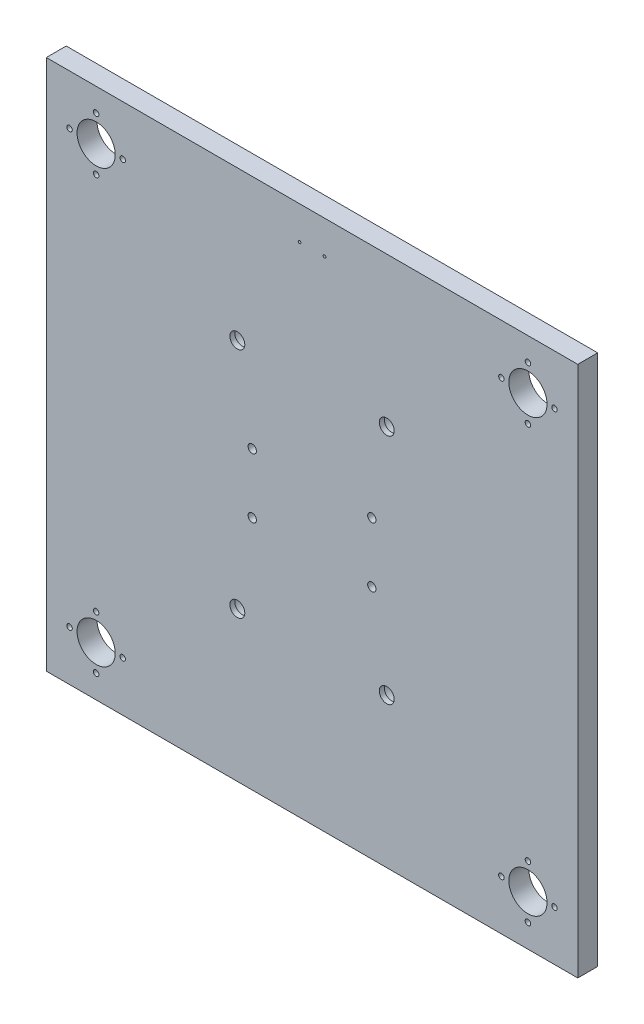
SolidWorks part; units mm, degrees
material "6061 合金"
ref_plane "前视基准面" through (0, 0, 0) normal (0, 0, 1) x (1, 0, 0)
ref_plane "上视基准面" through (0, 0, 0) normal (0, 1, 0) x (1, 0, 0)
ref_plane "右视基准面" through (0, 0, 0) normal (1, 0, 0) x (0, 0, -1)
sketch "草图1" plane through (0, 0, 0) normal (0, 0, 1) x (1, 0, 0)
  line L1 (-160, 160) -> (160, 160)
  line L2 (-160, 160) -> (-160, -160)
  line L3 (-160, -160) -> (160, -160)
  line L4 (160, 160) -> (160, -160)
  line L5 (-160, 160) -> (160, -160) construction
  line L6 (-160, -160) -> (160, 160) construction
  circle A0 centre (-130, 130) radius 11.5
  circle A1 centre (130, 130) radius 11.5
  circle A2 centre (130, -130) radius 11.5
  circle A3 centre (-130, -130) radius 11.5
  point P0 (0, 0)
  point P17 (0, 0)
  dimension "D3" = 23
  dimension "D7" = 30
  dimension "D8" = 30
  dimension "D1" = 320
  dimension "D2" = 320
  dimension "D4" = 30
  dimension "D6" = 30
  dimension "D5" = 4
extrude "凸台-拉伸1" add sketch "草图1" along normal mid plane 12
hole_wizard "M6 螺纹孔1" positions "草图3" profile "草图2" tap size "M6" standard "GB" end condition through all
sketch "草图3" plane through (0, 0, -6) normal (0, 0, -1) x (-1, 0, 0)
  point P0 (-36, 18)
  point P2 (-36, -18)
  point P4 (36, -18)
  point P6 (36, 18)
  dimension "D1" = 72
  dimension "D2" = 36
  dimension "D3" = 36
  dimension "D4" = 18
sketch "草图2" plane through (36, 18, -6) normal (1, 0, 0) x (0, 1, 0)
  line L0 (0, 0) -> (0, 12)
  line L1 (0, 12) -> (2.5, 12)
  line L2 (2.5, 12) -> (2.5, 0)
  line L5 (2.5, 0) -> (0, 0)
  line L11 (0, -6.35) -> (0, 107.95) construction
  dimension "通孔螺纹孔钻头直径" = 5
  dimension "通孔螺纹孔钻头深度" = 12
cosmetic thread "孔螺蚊线1" parameters "D2"=6
cosmetic thread "孔螺蚊线2" parameters "D2"=6
cosmetic thread "孔螺蚊线3" parameters "D2"=6
cosmetic thread "孔螺蚊线4" parameters "D2"=6
hole_wizard "打孔尺寸(%根据)内六角圆柱头螺钉的类型1" positions "草图5" profile "草图4" counterbore size "M8" standard "GB" end condition through all
sketch "草图5" plane through (0, 0, -6) normal (0, 0, -1) x (-1, 0, 0)
  point P0 (-45, 70)
  point P2 (45, 70)
  point P4 (45, -70)
  point P6 (-45, -70)
  dimension "D1" = 90
  dimension "D2" = 140
  dimension "D3" = 70
  dimension "D4" = 45
sketch "草图4" plane through (45, 70, -6) normal (1, 0, 0) x (0, 1, 0)
  line L0 (0, 0) -> (0, 12)
  line L1 (0, 12) -> (4.5, 12)
  line L3 (4.5, 12) -> (4.5, 9)
  line L4 (4.5, 9) -> (7.5, 9)
  line L5 (7.5, 9) -> (7.5, 0)
  line L7 (7.5, 0) -> (0, 0)
  line L11 (0, -6.35) -> (0, 107.95) construction
  dimension "通孔孔直径" = 9
  dimension "通孔孔深度" = 12
  dimension "柱形沉头孔直径" = 15
  dimension "柱形沉头孔深度" = 9
hole_wizard "M4 螺纹孔2" positions "草图7" profile "草图8" tap size "M4" standard "GB" end condition through all
sketch "草图7" plane through (0, 0, 6) normal (0, 0, 1) x (1, 0, 0)
  circle A0 centre (-130, 130) radius 16
  point P0 (-130, 146)
  point P2 (-114, 130)
  point P4 (-130, 114)
  point P6 (-146, 130)
  dimension "D1" = 32
sketch "草图8" plane through (-130, 146, 6) normal (1, 0, 0) x (0, -1, 0)
  line L0 (0, 0) -> (0, 12)
  line L1 (0, 12) -> (1.65, 12)
  line L2 (1.65, 12) -> (1.65, 0)
  line L5 (1.65, 0) -> (0, 0)
  line L11 (0, -6.35) -> (0, 107.95) construction
  dimension "通孔螺纹孔钻头直径" = 3.3
  dimension "通孔螺纹孔钻头深度" = 12
cosmetic thread "孔螺蚊线5" parameters "D2"=4
cosmetic thread "孔螺蚊线6" parameters "D2"=4
cosmetic thread "孔螺蚊线7" parameters "D2"=4
cosmetic thread "孔螺蚊线8" parameters "D2"=4
mirror "镜向1" about plane through (0, 0, 0) normal (0, 1, 0) of "M4 螺纹孔2"
mirror "镜向2" about plane through (0, 0, 0) normal (1, 0, 0) of "镜向1", "M4 螺纹孔2"
hole_wizard "M4 螺纹孔1" positions "草图10" profile "草图9" tap size "M4" standard "GB"
sketch "草图10" plane through (0, 0, -6) normal (0, 0, -1) x (-1, 0, 0)
  line L0 (-160, 160) -> (160, 160) construction
  point P0 (-7.5, 140)
  point P2 (7.5, 140)
  dimension "D1" = 15
  dimension "D2" = 20
  dimension "D3" = 7.5
sketch "草图9" plane through (7.5, 140, -6) normal (1, 0, 0) x (0, 1, 0)
  line L0 (0, 0) -> (0, 12.4914)
  line L1 (0, 12.4914) -> (1.65, 11.5)
  line L2 (1.65, 11.5) -> (1.65, 0)
  line L5 (1.65, 0) -> (0, 0)
  line L10 (0, 12.4914) -> (-1.65, 11.5) construction
  line L11 (0, -6.35) -> (0, 107.95) construction
  dimension "螺纹孔钻头直径" = 3.3
  dimension "螺纹孔钻头深度" = 11.5
  dimension "导头角度" = 118
cosmetic thread "孔螺蚊线9" parameters "D1"=8, "D2"=4
cosmetic thread "孔螺蚊线10" parameters "D1"=8, "D2"=4
